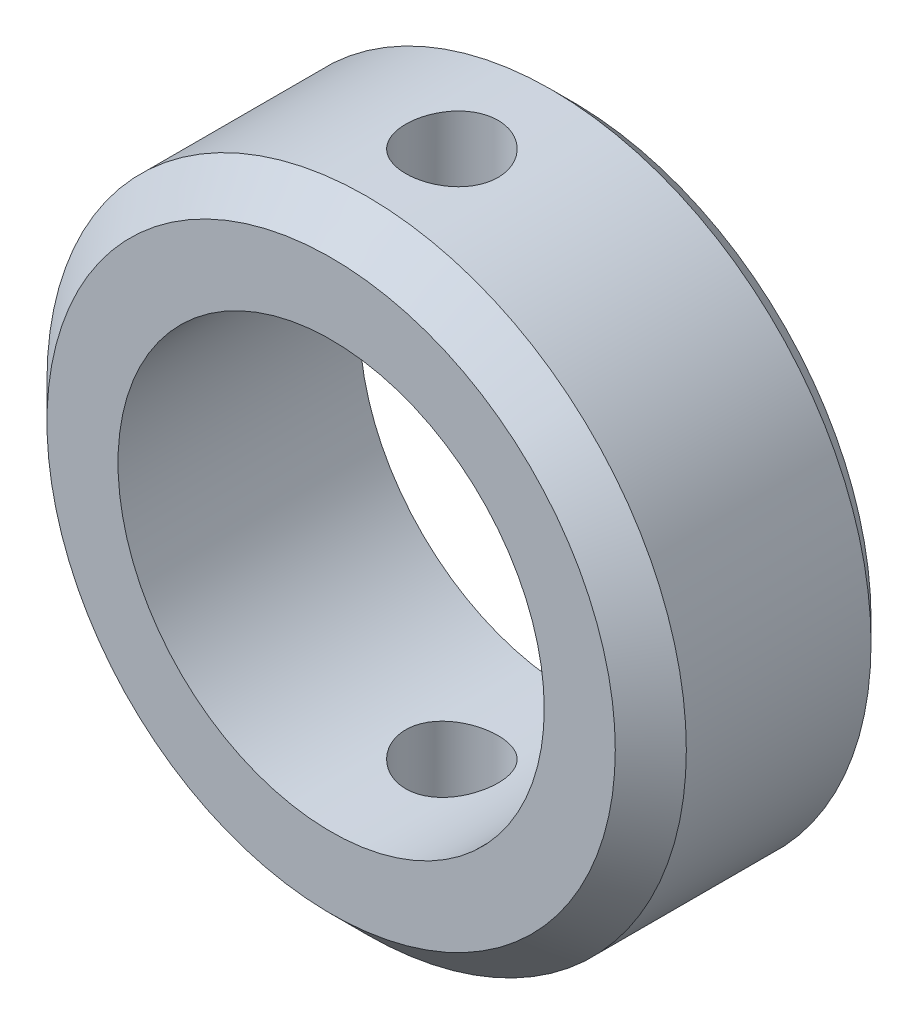
SolidWorks part; units mm, degrees
ref_plane "Front Plane" through (0, 0, 0) normal (0, 0, 1) x (1, 0, 0)
ref_plane "Top Plane" through (0, 0, 0) normal (0, 1, 0) x (1, 0, 0)
ref_plane "Right Plane" through (0, 0, 0) normal (1, 0, 0) x (0, 0, -1)
sketch "Sketch1" plane through (0, 0, 0) normal (0, 0, 1) x (1, 0, 0)
  circle A0 centre (0, 0) radius 30
  circle A1 centre (0, 0) radius 45
  dimension "D1" = 60
  dimension "D2" = 90
extrude "Boss-Extrude1" add sketch "Sketch1" along normal blind 34
sketch "Sketch3" plane through (0, 0, 0) normal (0, 1, 0) x (1, 0, 0)
  line L0 (-30, -34) -> (30, -34) construction
  line L1 (0, 0) -> (0, -40.3636) construction
  circle A0 centre (0, -17) radius 6.5
  dimension "D2" = 13
  dimension "D1" = 17
extrude "Cut-Extrude1" cut sketch "Sketch3" against normal through all and the other way through all
chamfer "Chamfer1" distance 5 angle 45 1 edges at (45, 0, 34)
chamfer "Chamfer2" distance 3 angle 45 1 edges at (45, 0, 0)
